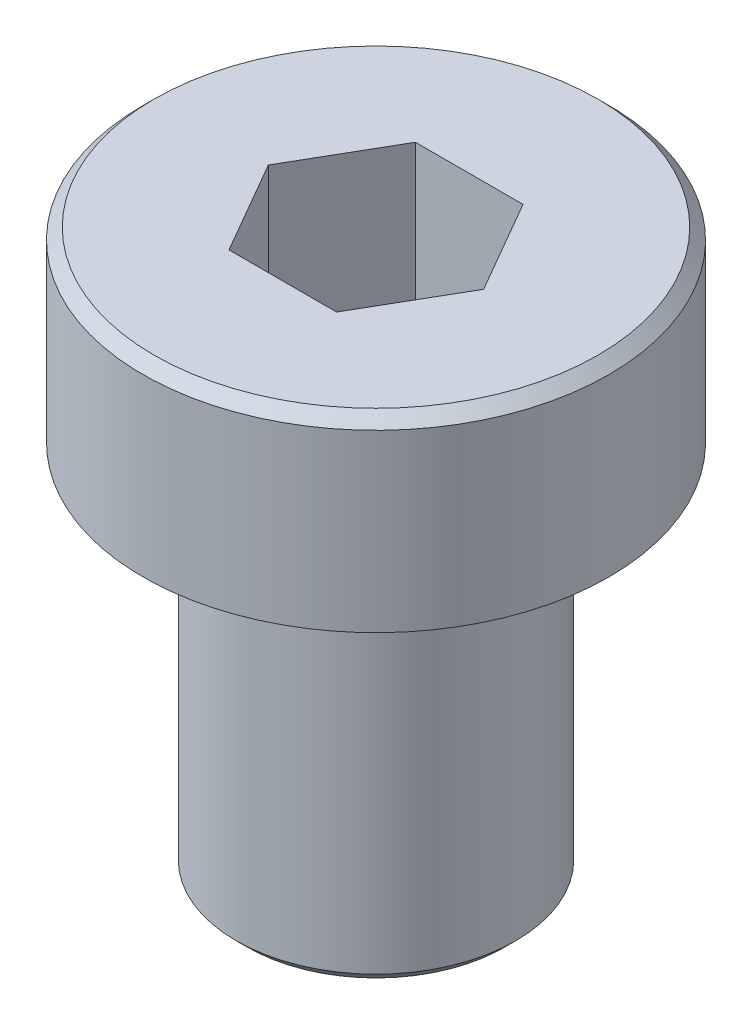
SolidWorks part; units mm, degrees
ref_plane "Front Plane" through (0, 0, 0) normal (0, 0, 1) x (1, 0, 0)
ref_plane "Top Plane" through (0, 0, 0) normal (0, 1, 0) x (1, 0, 0)
ref_plane "Right Plane" through (0, 0, 0) normal (1, 0, 0) x (0, 0, -1)
sketch "Sketch1" plane through (0, 0, 0) normal (0, 0, 1) x (1, 0, 0)
  line L0 (0, 0) -> (0, 8) construction
  line L1 (3, 0) -> (5, 0)
  line L2 (3, 0) -> (3, 8)
  line L3 (3, 8) -> (0, 8)
  line L6 (2, -4) -> (2, -1)
  line L7 (2, -1) -> (0, 0.1547)
  line L11 (3, 0) -> (5, 0)
  line L12 (5, 0) -> (5, -4)
  line L13 (5, -4) -> (0, -4)
  point P7 (3, 0)
  dimension "D1" = 60
  dimension "M" = 6
  dimension "L" = 8
  dimension "t" = 3
  dimension "B" = 4
  dimension "E" = 4
  dimension "A" = 10
  dimension "(l)" = 8
sketch "Sketch2" plane through (0, 0, 0) normal (0, 0, 1) x (1, 0, 0)
  line L0 (2, -4) -> (2, -1) construction
  line L1 (2, -1) -> (0, 0.1547) construction
  line L3 (3, 0) -> (3, 8) construction
  line L4 (3, 0) -> (5, 0) construction
  line L7 (2, -4) -> (2, -1)
  line L8 (2, -1) -> (0, 0.1547)
  line L9 (5, 0) -> (5, -4) construction
  line L10 (3, 0) -> (3, 8)
  line L14 (0, 0.1547) -> (0, 8)
  line L16 (3, 8) -> (0, 8) construction
  line L19 (3, 8) -> (0, 8)
  line L20 (5, -4) -> (0, -4) construction
  line L21 (3, 0) -> (5, 0)
  line L22 (5, 0) -> (5, -4)
  line L23 (5, -4) -> (2, -4)
revolve "Revolve1" add sketch "Sketch2" angle 360 mid plane about L14
cosmetic thread "Cosmetic Thread1" parameters "D1"=8, "D2"=5.28
chamfer "Chamfer1" distance 0.24 angle 45 2 edges at (3, 8, 0) (5, -4, 0)
sketch "Sketch3" plane through (0, -4, 0) normal (0, -1, 0) x (1, 0, 0)
  line L1 (-1.1547, 2) -> (-2.3094, 0)
  line L2 (-2.3094, 0) -> (-1.1547, -2)
  line L3 (-1.1547, -2) -> (1.1547, -2)
  line L4 (1.1547, -2) -> (2.3094, 0)
  line L5 (2.3094, 0) -> (1.1547, 2)
  line L6 (1.1547, 2) -> (-1.1547, 2)
  circle A0 centre (0, 0) radius 2 construction
extrude "Cut-Extrude1" cut sketch "Sketch3" against normal up to vertex (3 mm away) up to point (2, -1, 0)
move or copy body "Body-Move/Copy1" bodies to move or copy 102 copy no rotation origin (0, 3.25, 0) rotation axis (1, 0, 0) rotation angle 180
